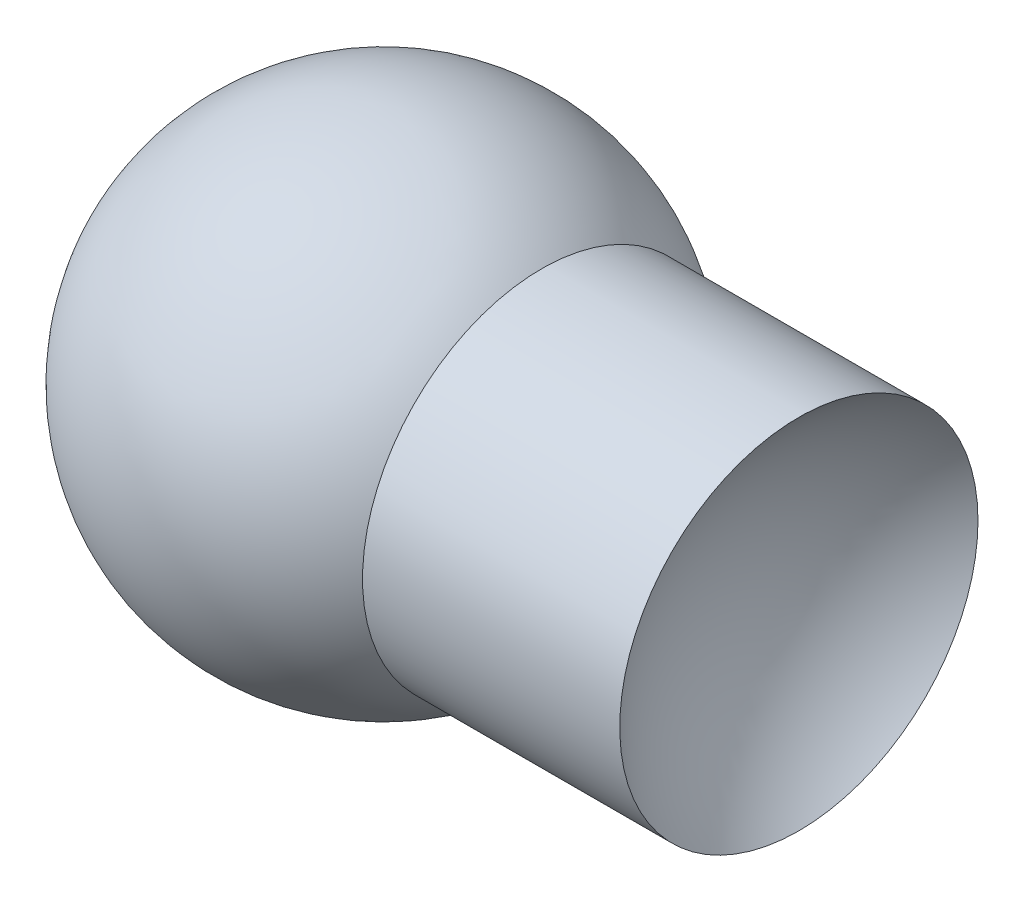
from build123d import *


with BuildPart() as part:
    # Sketch1 → Revolve3 (revolve)
    with BuildSketch(Plane.XY):
        with BuildLine():
            Line((0, 10), (0, -10))
            ThreePointArc((0, -10), (10, 0), (0, 10))
        make_face()
    revolve(axis=Axis((0, 23.790519838, 0), (0, -1, 0)))

    # Sketch2 → Revolve4 (revolve)
    with BuildSketch(Plane.XY, mode=Mode.PRIVATE) as revolve4_sk:
        with BuildLine():
            Line((6.614378278, 7.5), (17.385621722, 7.5))
            ThreePointArc((17.385621722, 7.5), (14.885621722, 4.114378278), (14, 0))
            Line((14, 0), (10, 0))
            ThreePointArc((10, 0), (9.114378278, 4.114378278), (6.614378278, 7.5))
        make_face()
    revolve(revolve4_sk.sketch.rotate(Axis((27.637994168, 0, 0), (-1, 0, 0)), 90), axis=Axis((27.637994168, 0, 0), (-1, 0, 0)))


solid = part.part
